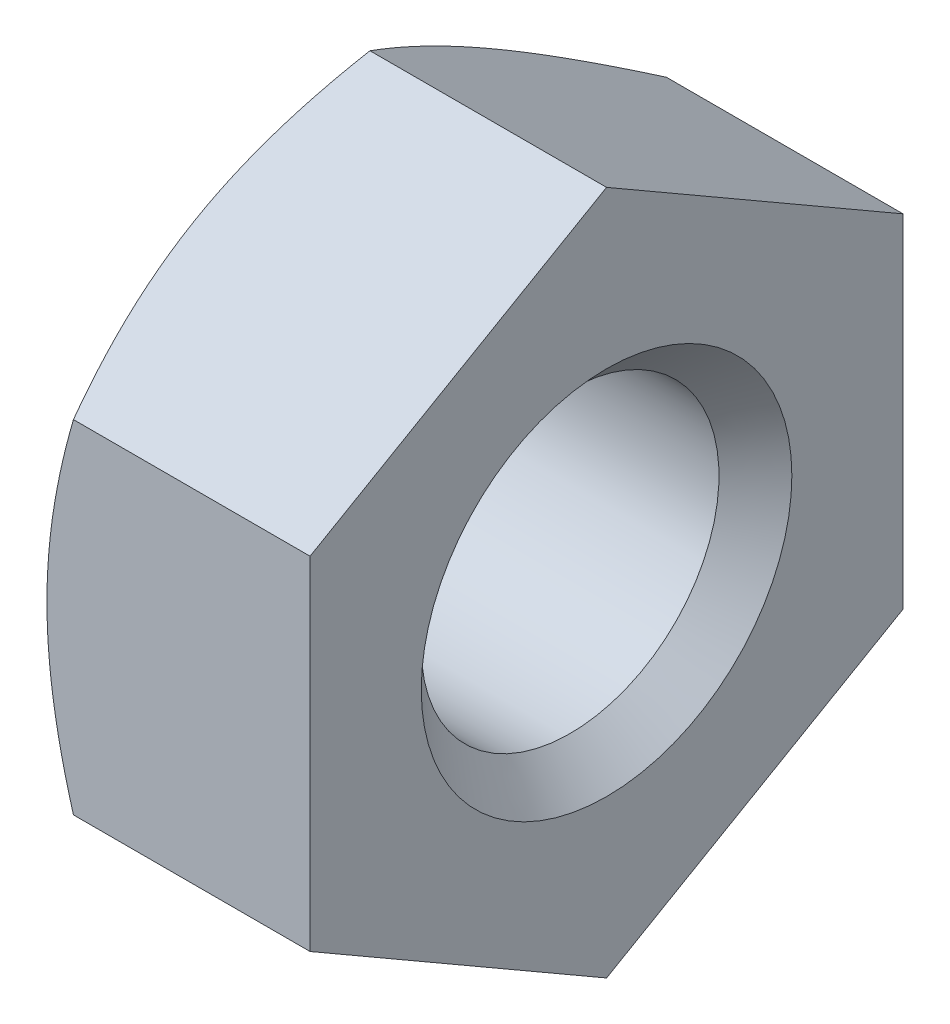
from build123d import *

# Parameters (mm, degrees)
SKETCH3_W          = 16
SKETCH3_H          = 16
CUT_EXTRUDE1_DEPTH = 4


with BuildPart() as part:
    # Sketch1 → Revolve1 (revolve)
    with BuildSketch(Plane.XY, mode=Mode.PRIVATE) as revolve1_sk:
        Polygon((-4, 0), (-4, 3.22), (-2.937675505, 5.06), (0, 5.06), (0, 0), align=None)
    revolve(revolve1_sk.sketch.rotate(Axis((0, 0, 0), (-1, 0, 0)), 270), axis=Axis((0, 0, 0), (-1, 0, 0)))

    # Sketch2 → Cut-Revolve1 (revolve, cut)
    with BuildSketch(Plane.XY, mode=Mode.PRIVATE) as cut_revolve1_sk:
        Polygon((-4, 0), (-4, 2.5), (-3.508532, 2.008532), (-0.491468, 2.008532), (0, 2.5), (0, 0), align=None)
    revolve(cut_revolve1_sk.sketch.rotate(Axis((0, 0, 0), (-1, 0, 0)), 270), axis=Axis((0, 0, 0), (-1, 0, 0)), mode=Mode.SUBTRACT)

    # Sketch3 → Cut-Extrude1 (cut)
    with BuildSketch(Plane(origin=(0, 0, 0), x_dir=(0, 0, -1), z_dir=(1, 0, 0))):
        Rectangle(SKETCH3_W, SKETCH3_H)
        Polygon((-4, 2.309401077), (-4, -2.309401077), (0, -4.618802154), (4, -2.309401077), (4, 2.309401077), (0, 4.618802154), align=None, mode=Mode.SUBTRACT)
    extrude(amount=-CUT_EXTRUDE1_DEPTH, mode=Mode.SUBTRACT)


solid = part.part
